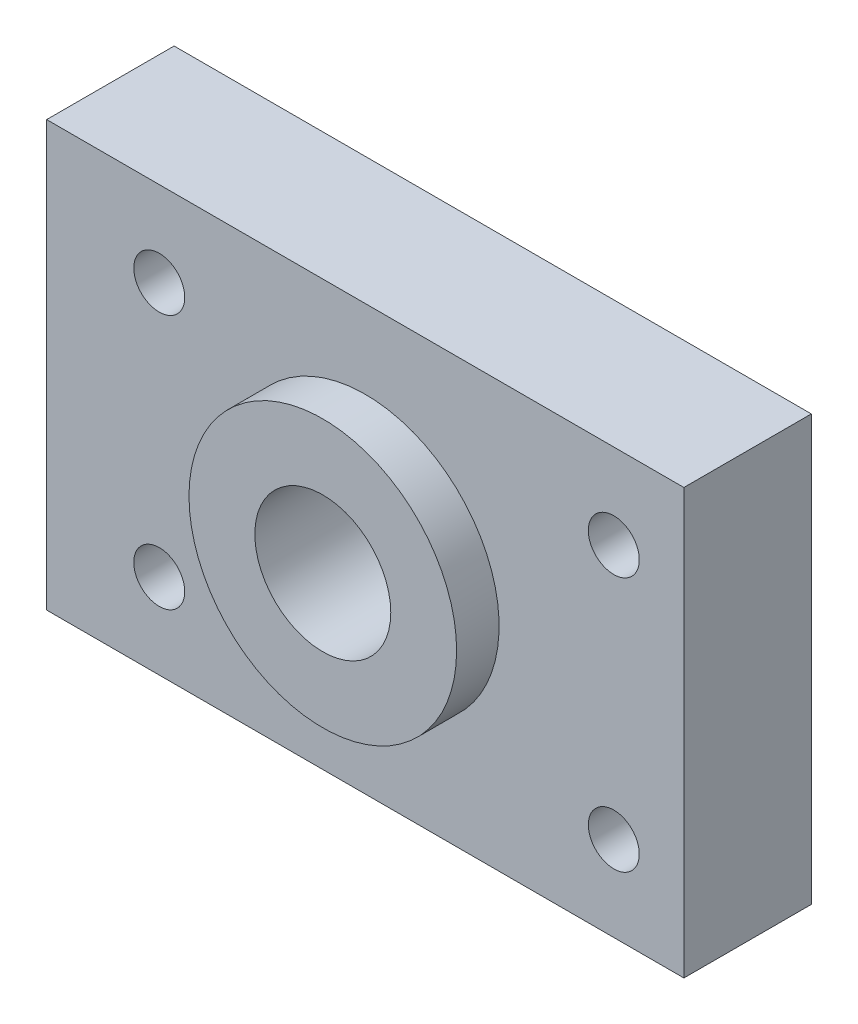
SolidWorks part; units mm, degrees
ref_plane "前视基准面" through (0, 0, 0) normal (0, 0, 1) x (1, 0, 0)
ref_plane "上视基准面" through (0, 0, 0) normal (0, 1, 0) x (1, 0, 0)
ref_plane "右视基准面" through (0, 0, 0) normal (1, 0, 0) x (0, 0, -1)
other "Configuration Table"
sketch "草图1" plane through (0, 0, 0) normal (0, 0, 1) x (1, 0, 0)
  line L1 (-75, -50) -> (75, -50)
  line L2 (-75, -50) -> (-75, 50)
  line L3 (-75, 50) -> (75, 50)
  line L4 (75, -50) -> (75, 50)
  line L5 (0, 50) -> (0, -50) construction
  line L6 (-75, 0) -> (75, 0) construction
  point P0 (0, 0)
  dimension "D1" = 100
  dimension "D2" = 150
extrude "凸台-拉伸1" add sketch "草图1" along normal blind 30
sketch "草图2" plane through (0, 0, 30) normal (0, 0, 1) x (1, 0, 0)
  circle A0 centre (0, 0) radius 31.5
  circle A1 centre (0, 0) radius 16
  dimension "D1" = 63
  dimension "D2" = 32
extrude "凸台-拉伸2" add sketch "草图2" along normal blind 10
sketch "草图3" plane through (0, 0, 30) normal (0, 0, 1) x (1, 0, 0)
  circle A1 centre (0, 0) radius 16
  circle A2 centre (0, 0) radius 16
  dimension "D1" = 0
extrude "切除-拉伸1" cut sketch "草图3" against normal through all
sketch "草图4" plane through (0, 0, 0) normal (0, 0, -1) x (-1, 0, 0)
  line L0 (-75, 50) -> (75, 50) construction
  line L1 (-58.5, -30) -> (58.5, -30) construction
  line L5 (0, 30) -> (0, -30) construction
  line L6 (-58.5, 0) -> (58.5, 0) construction
  circle A0 centre (-58.5, 30) radius 6
  circle A1 centre (48.5, 30) radius 6
  circle A2 centre (48.5, -30) radius 6
  circle A3 centre (-58.5, -30) radius 6
  point P0 (0, 0)
  dimension "D3" = 12
  dimension "D8" = 58.5
  dimension "D1" = 58.5
  dimension "D2" = 60
  dimension "D6" = 107
  dimension "D7" = 20
  dimension "D9" = 107
  dimension "D4" = 2
  dimension "D5" = 2
extrude "切除-拉伸2" cut sketch "草图4" against normal through all
